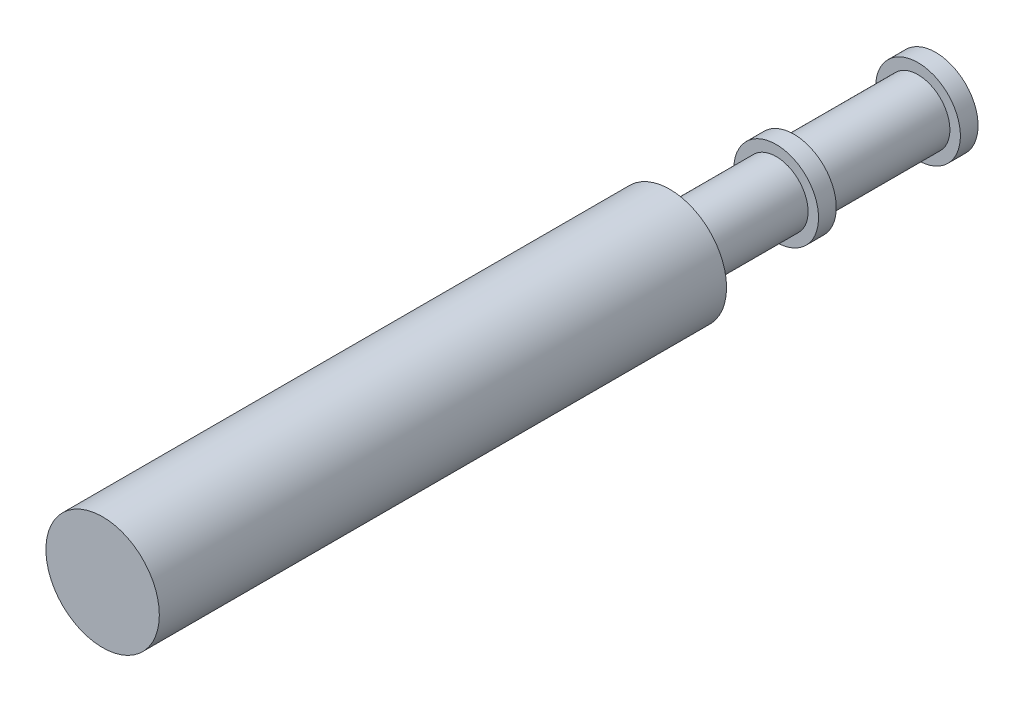
SolidWorks part; units mm, degrees
other "Annotation1"
sketch "草图4" plane through (-44.545, -92.366, -398.1258) normal (-0.5802, -0.6393, -0.5046) x (0.2397, -0.7262, 0.6444)
ref_plane "Front Plane" through (0, 0, 0) normal (0, 0, 1) x (1, 0, 0)
ref_plane "Top Plane" through (0, 0, 0) normal (0, 1, 0) x (1, 0, 0)
ref_plane "Right Plane" through (0, 0, 0) normal (1, 0, 0) x (0, 0, -1)
sketch "Sketch5" plane through (0, 0, 0) normal (0, 0, 1) x (1, 0, 0)
  circle A0 centre (-19.201, 5.8685) radius 16
  dimension "D1" = 32
extrude "Boss-Extrude1" add sketch "Sketch5" against normal blind 60 separate body
sketch "Sketch6" plane through (0, 0, -60) normal (0, 0, -1) x (-1, 0, 0)
  circle A0 centre (19.201, 5.8685) radius 9
  dimension "D1" = 18
extrude "Boss-Extrude2" add sketch "Sketch6" along normal blind 70
sketch "Sketch7" plane through (0, 0, 0) normal (0, 0, 1) x (1, 0, 0)
  circle A0 centre (-19.201, 5.8685) radius 16
extrude "Boss-Extrude3" add sketch "Sketch7" along normal blind 100
sketch "Sketch8" plane through (0, 0, -130) normal (0, 0, -1) x (-1, 0, 0)
  circle A0 centre (19.201, 5.8685) radius 11.9522
extrude "Boss-Extrude4" add sketch "Sketch8" along normal blind 5
pattern_linear "LPattern1" count 2 spacing 40 along (0, 0, 1) of "Boss-Extrude4"
